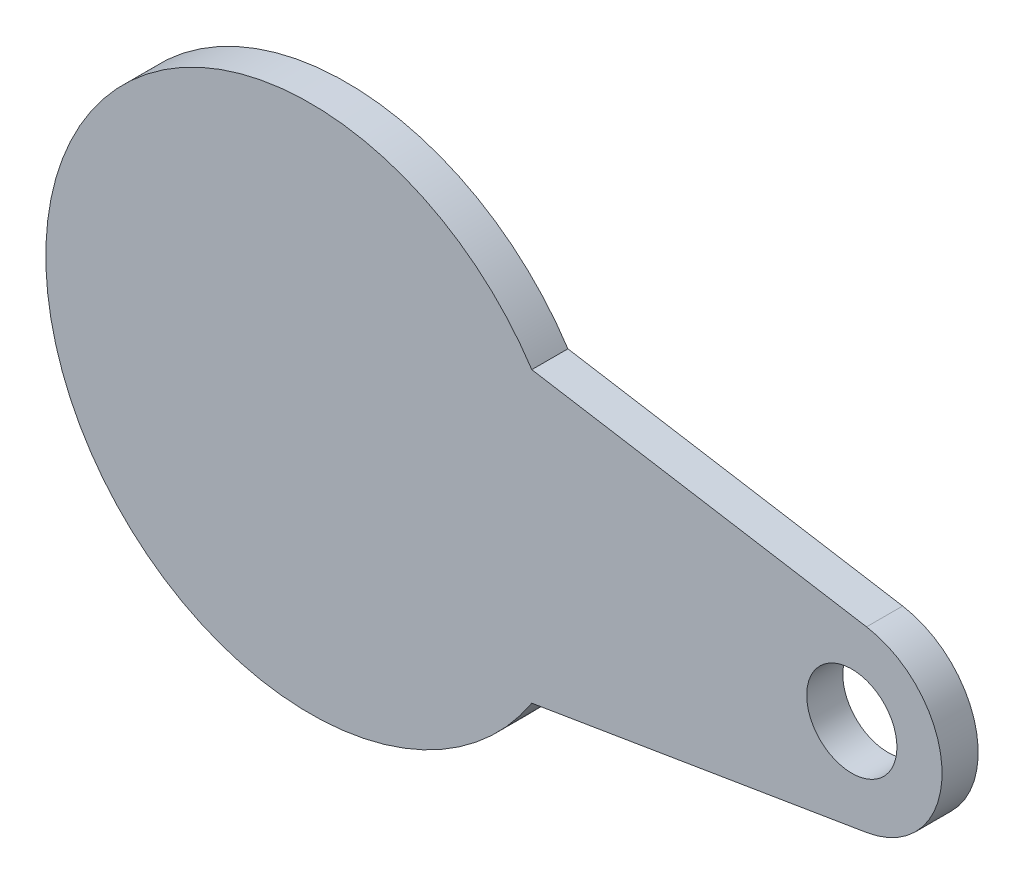
from build123d import *

# Parameters (mm, degrees)
SKETCH1_R           = 25
BOSS_EXTRUDE1_DEPTH = 20


with BuildPart() as part:
    # Sketch1 → Boss-Extrude1 (new body)
    with BuildSketch(Plane.XY):
        with BuildLine():
            Line((122.728358581, 80), (308.159136141, 49.329793203))
            ThreePointArc((308.159136141, 49.329793203), (350, 0), (308.159136141, -49.329793203))
            Line((308.159136141, -49.329793203), (122.728358581, -80))
            ThreePointArc((122.728358581, -80), (-146.5, 0), (122.728358581, 80))
        make_face()
        with Locations((300, 0)):
            Circle(SKETCH1_R, mode=Mode.SUBTRACT)
    extrude(amount=BOSS_EXTRUDE1_DEPTH)


solid = part.part
